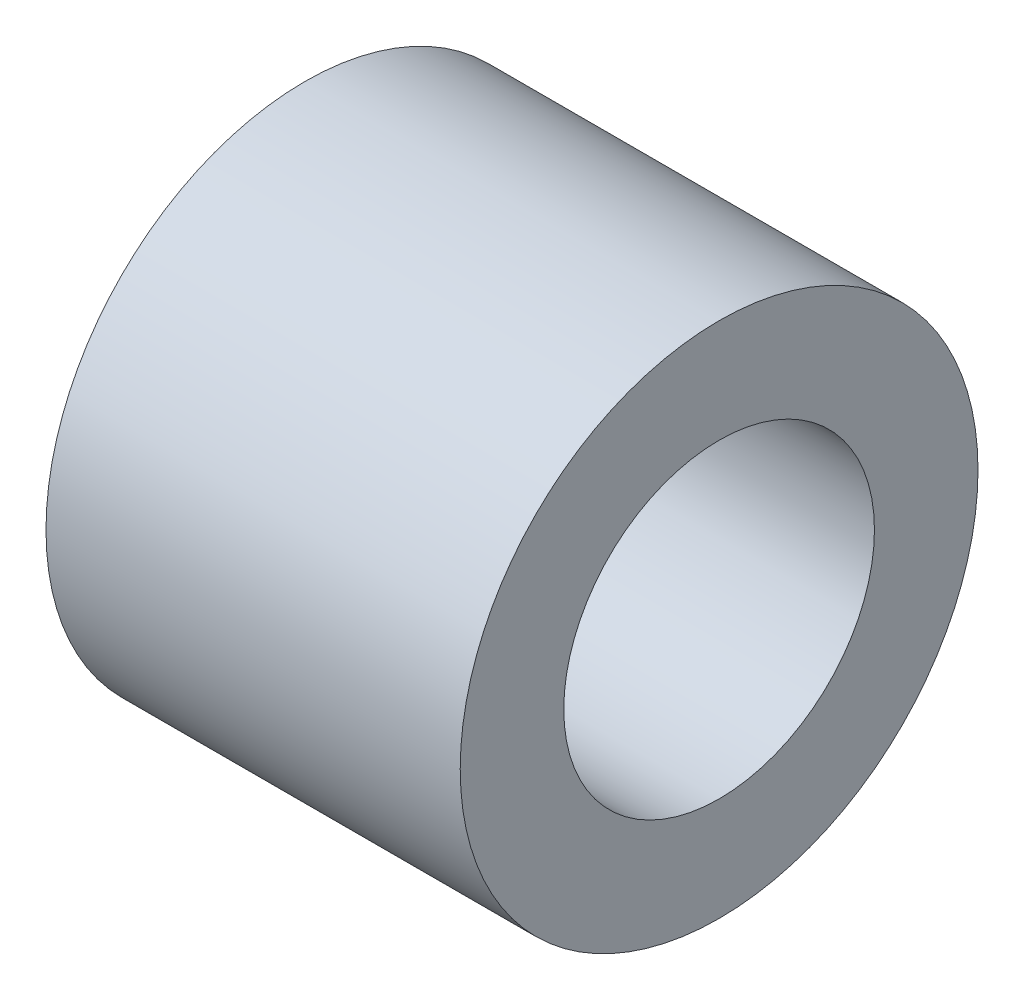
from build123d import *

# Parameters (mm, degrees)
SKETCH_1_R                = 12.5
EXTRUDE_1_DEPTH           = 20
HOLE_WIZARD_1_D           = 9
HOLE_WIZARD_1_CBORE_D     = 15
HOLE_WIZARD_1_CBORE_DEPTH = 12


with BuildPart() as part:
    # 草图1 → 凸台-拉伸1 (new body)
    with BuildSketch(Plane(origin=(0, 0, 0), x_dir=(0, 0, -1), z_dir=(1, 0, 0))):
        Circle(SKETCH_1_R)
    extrude(amount=EXTRUDE_1_DEPTH)

    # 打孔尺寸(%根据)内六角圆柱头螺钉的类型1 (through all)
    with Locations(Plane(origin=(20, 0, 0), x_dir=(0, 0, -1), z_dir=(1, 0, 0))):
        with Locations((0, 0)):
            CounterBoreHole(HOLE_WIZARD_1_D / 2, HOLE_WIZARD_1_CBORE_D / 2, HOLE_WIZARD_1_CBORE_DEPTH)


solid = part.part
